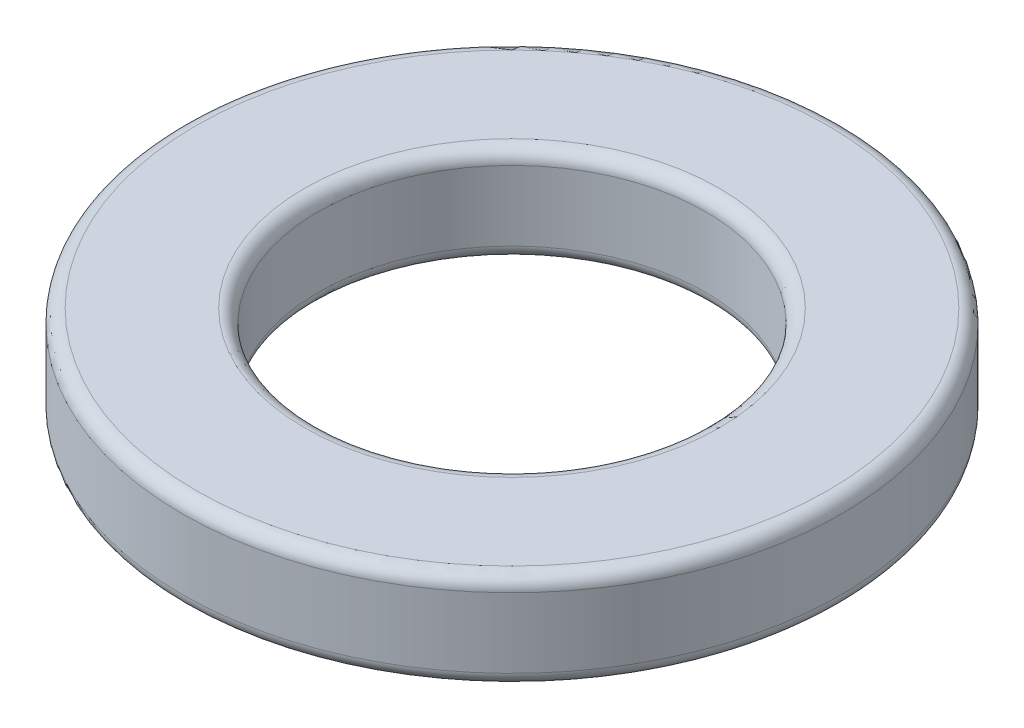
from build123d import *

# Parameters (mm, degrees)
SKETCH_1_R      = 1.7
SKETCH_1_R_2    = 1
EXTRUDE_1_DEPTH = 0.5
FILLET_1_R      = 0.07


with BuildPart() as part:
    # 草图1 → 凸台-拉伸1 (new body)
    with BuildSketch(Plane(origin=(0, 0, 0), x_dir=(1, 0, 0), z_dir=(0, 1, 0))):
        with Locations(Location((0, 0, 0), (0, 0, 270))):
            Circle(SKETCH_1_R)
        with Locations(Location((0, 0, 0), (0, 0, 270))):
            Circle(SKETCH_1_R_2, mode=Mode.SUBTRACT)
    extrude(amount=EXTRUDE_1_DEPTH)

    # 圆角1
    fillet_1_edges = [part.edges().sort_by_distance(p)[0] for p in [
        (0, 0, -1.7),
        (0, 0.5, -1.7),
        (0, 0, -1),
        (0, 0.5, -1),
    ]]
    fillet(fillet_1_edges, radius=FILLET_1_R)


solid = part.part
